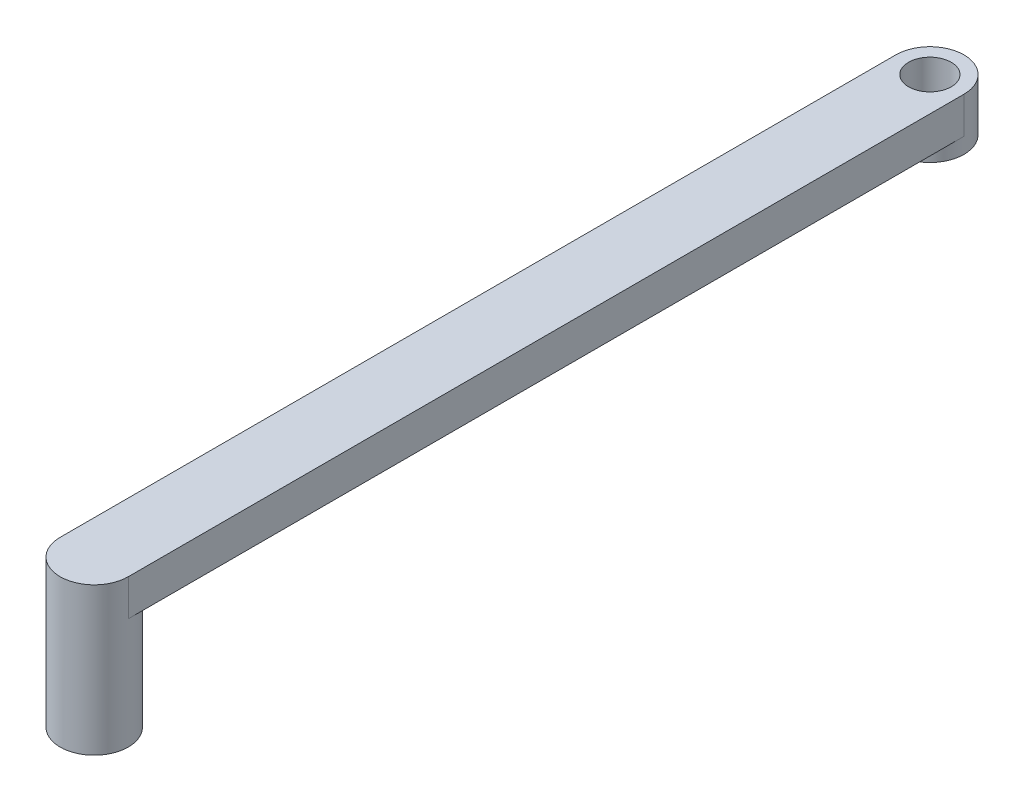
SolidWorks part; units mm, degrees
ref_plane "Front Plane" through (0, 0, 0) normal (0, 0, 1) x (1, 0, 0)
ref_plane "Top Plane" through (0, 0, 0) normal (0, 1, 0) x (1, 0, 0)
ref_plane "Right Plane" through (0, 0, 0) normal (1, 0, 0) x (0, 0, -1)
sketch "Sketch1" plane through (0, 0, 0) normal (0, 1, 0) x (1, 0, 0)
  circle A0 centre (0, 0) radius 125
  circle A1 centre (0, 0) radius 200
  dimension "D1" = 250
  dimension "D2" = 400
extrude "Boss-Extrude1" add sketch "Sketch1" against normal blind 220
sketch "Sketch2" plane through (0, 0, 0) normal (0, 1, 0) x (1, 0, 0)
  line L0 (-200, 0) -> (-200, -4903.055)
  line L1 (0, 772.8443) -> (0, -1449.9063) construction
  line L2 (200, 0) -> (200, -4903.055)
  circle A0 centre (0, 0) radius 200 construction
  circle A1 centre (0, -4903.055) radius 200
  arc A2 (-200, 0) -> (200, 0) centre (0, 0) ccw
  dimension "D1" = 4903.055
extrude "Boss-Extrude2" add sketch "Sketch2" against normal blind 214
sketch "Sketch3" plane through (0, 0, 0) normal (0, 1, 0) x (1, 0, 0)
  circle A0 centre (0, -4903.055) radius 200
extrude "Boss-Extrude3" add sketch "Sketch3" against normal blind 780
sketch "Sketch4" plane through (0, -780, 0) normal (0, -1, 0) x (1, 0, 0)
  circle A0 centre (0, 4903.055) radius 137.5
  dimension "D1" = 275
extrude "Cut-Extrude1" cut sketch "Sketch4" against normal blind 604
sketch "Sketch5" plane through (0, -780, 0) normal (0, -1, 0) x (1, 0, 0)
  circle A0 centre (0, 4903.055) radius 200
  circle A1 centre (0, 4903.055) radius 90
  dimension "D1" = 180
extrude "Boss-Extrude4" add sketch "Sketch5" along normal blind 86
sketch "Sketch6" plane through (0, -220, 0) normal (0, -1, 0) x (1, 0, 0)
  circle A0 centre (0, 0) radius 200
extrude "Boss-Extrude5" add sketch "Sketch6" along normal blind 86
